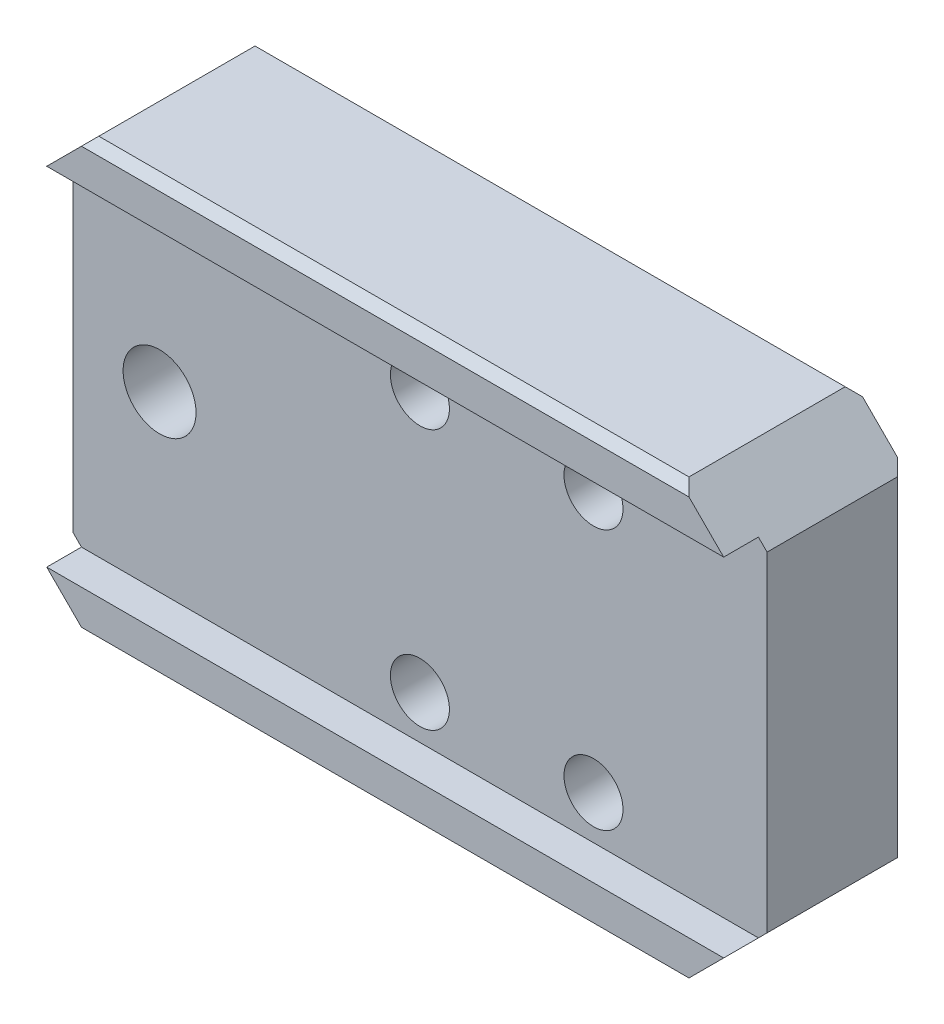
SolidWorks part; units mm, degrees
material "A6061"
ref_plane "Front Plane" through (0, 0, 0) normal (0, 0, 1) x (1, 0, 0)
ref_plane "Top Plane" through (0, 0, 0) normal (0, 1, 0) x (1, 0, 0)
ref_plane "Right Plane" through (0, 0, 0) normal (1, 0, 0) x (0, 0, -1)
sketch "Sketch1" plane through (0, 0, 0) normal (0, 0, 1) x (1, 0, 0)
  line L1 (-20, -12.5) -> (20, -12.5)
  line L2 (-20, -12.5) -> (-20, 12.5)
  line L3 (-20, 12.5) -> (20, 12.5)
  line L4 (20, -12.5) -> (20, 12.5)
  line L5 (-20, -12.5) -> (20, 12.5) construction
  line L6 (-20, 12.5) -> (20, -12.5) construction
  point P0 (0, 0)
  dimension "D1" = 40
  dimension "D2" = 25
extrude "Boss-Extrude1" add sketch "Sketch1" along normal blind 10
sketch "Sketch2" plane through (0, 0, 10) normal (0, 0, 1) x (1, 0, 0)
  line L0 (20, -12.5) -> (20, 12.5) construction
  line L1 (-20, -10) -> (20, -10)
  line L2 (-20, -10) -> (-20, 10)
  line L3 (-20, 10) -> (20, 10)
  line L4 (20, -10) -> (20, 10)
  line L5 (-20, -10) -> (20, 10) construction
  line L6 (-20, 10) -> (20, -10) construction
  point P0 (0, 0)
  dimension "D1" = 20
extrude "Cut-Extrude1" cut sketch "Sketch2" against normal blind 2
hole_wizard "M5 Tapped Hole1" positions "Sketch4" profile "Sketch3" tap size "M5" standard "GB" end condition through all
sketch "Sketch4" plane through (0, 0, 8) normal (0, 0, 1) x (1, 0, 0)
  line L0 (-20, 10) -> (-20, -10) construction
  point P0 (-15, 0)
  dimension "D1" = 5
cosmetic thread "Cosmetic Thread1" parameters "D2"=5
sketch "Sketch3" plane through (-15, 0, 8) normal (1, 0, 0) x (0, -1, 0)
  line L0 (0, 0) -> (0, 8)
  line L1 (0, 8) -> (2.1, 8)
  line L2 (2.1, 8) -> (2.1, 0)
  line L5 (2.1, 0) -> (0, 0)
  line L11 (0, -6.35) -> (0, 107.95) construction
  dimension "通孔螺纹孔钻头直径" = 4.2
  dimension "通孔螺纹孔钻头深度" = 8
hole_wizard "Hole Size (Based On) Socket Head Cap Screw Type1" positions "Sketch6" profile "Sketch5" counterbore size "M3" standard "GB" end condition through all
sketch "Sketch6" plane through (0, 0, 0) normal (0, 0, -1) x (-1, 0, 0)
  line L7 (20, 0) -> (-20, 0)
  line L8 (20, 12.5) -> (20, -12.5) construction
  line L9 (-20, -12.5) -> (-20, 12.5) construction
  line L12 (-10, 7.5) -> (0, 7.5)
  line L13 (-10, 7.5) -> (-10, -7.5)
  line L14 (-10, -7.5) -> (0, -7.5)
  line L15 (0, 7.5) -> (0, -7.5)
  point P0 (-10, 7.5)
  point P2 (-10, -7.5)
  point P4 (0, 7.5)
  point P6 (0, -7.5)
  dimension "D1" = 10
  dimension "D2" = 15
  dimension "D3" = 7.5
  dimension "D4" = 10
sketch "Sketch5" plane through (10, 7.5, 0) normal (1, 0, 0) x (0, 1, 0)
  line L0 (0, 0) -> (0, 10)
  line L1 (0, 10) -> (1.7, 10)
  line L3 (1.7, 10) -> (1.7, 3.4)
  line L4 (1.7, 3.4) -> (3, 3.4)
  line L5 (3, 3.4) -> (3, 0)
  line L7 (3, 0) -> (0, 0)
  line L11 (0, -6.35) -> (0, 107.95) construction
  dimension "通孔孔直径" = 3.4
  dimension "通孔孔深度" = 10
  dimension "柱形沉头孔直径" = 6
  dimension "柱形沉头孔深度" = 3.4
chamfer "Chamfer1" distance 3 angle 45 4 edges at (20, -12.5, 5) (20, 12.5, 5) (-20, -12.5, 5) (-20, 12.5, 5)
chamfer "Chamfer2" distance 0.5 angle 45 6 edges at (-20, 0, 0) (0, 12.5, 10) (0, 12.5, 0) (20, 0, 0) (0, -12.5, 10) (0, -12.5, 0)
